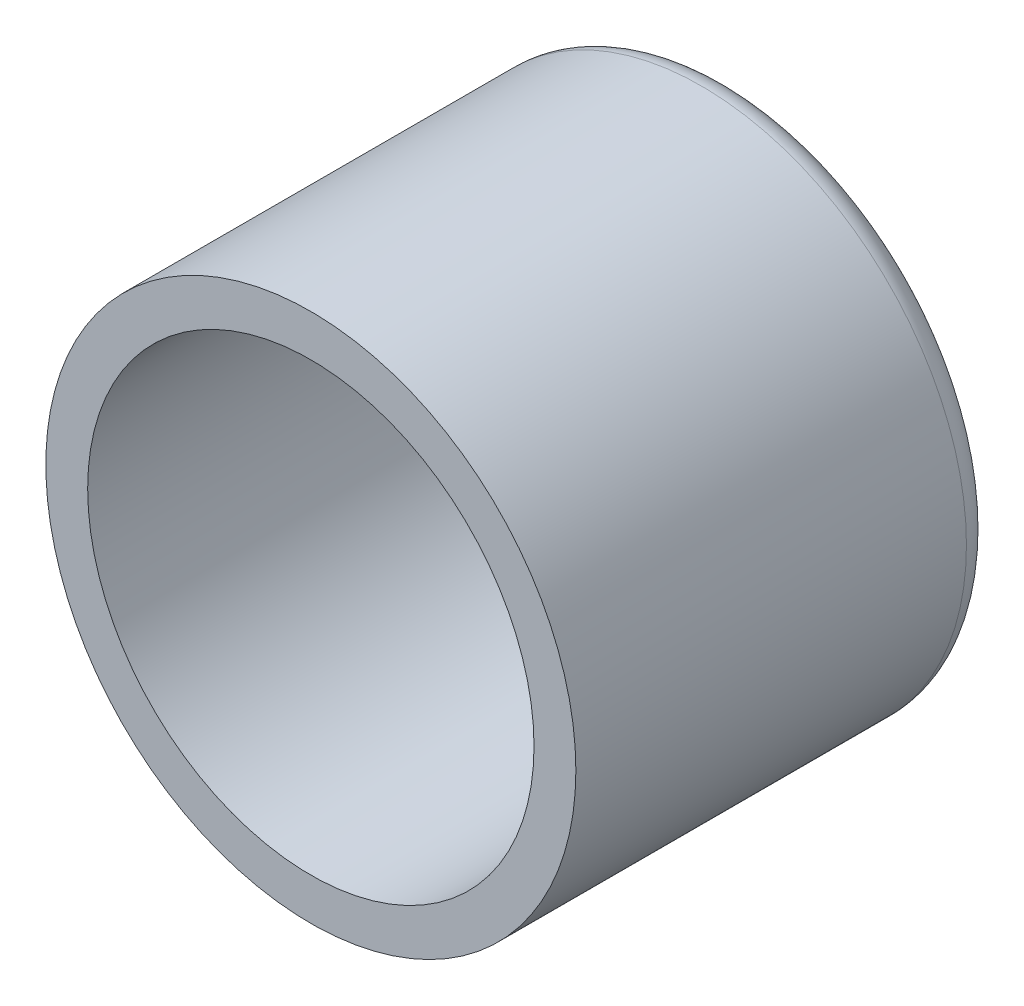
from build123d import *

# Parameters (mm, degrees)
BOSS_EXTRUDE1_DEPTH      = 100
BOSS_EXTRUDE1_DEPTH_BACK = 50
SKETCH1_R                = 95
SKETCH1_R_2              = 80
FILLET1_R                = 10


with BuildPart() as part:
    # Sketch1 → Boss-Extrude1 (new, two sides: drawn at the far end of the back side and taken through both)
    with BuildSketch(Plane.XY.offset(-BOSS_EXTRUDE1_DEPTH_BACK)):
        with Locations((-599.884196758, -90)):
            Circle(SKETCH1_R)
        with Locations((-599.884196758, -90)):
            Circle(SKETCH1_R_2, mode=Mode.SUBTRACT)
    extrude(amount=BOSS_EXTRUDE1_DEPTH + BOSS_EXTRUDE1_DEPTH_BACK)

    # Fillet1
    fillet1_edges = [part.edges().sort_by_distance(p)[0] for p in [
        (-694.884196758, -90, -50),
    ]]
    fillet(fillet1_edges, radius=FILLET1_R)


solid = part.part
